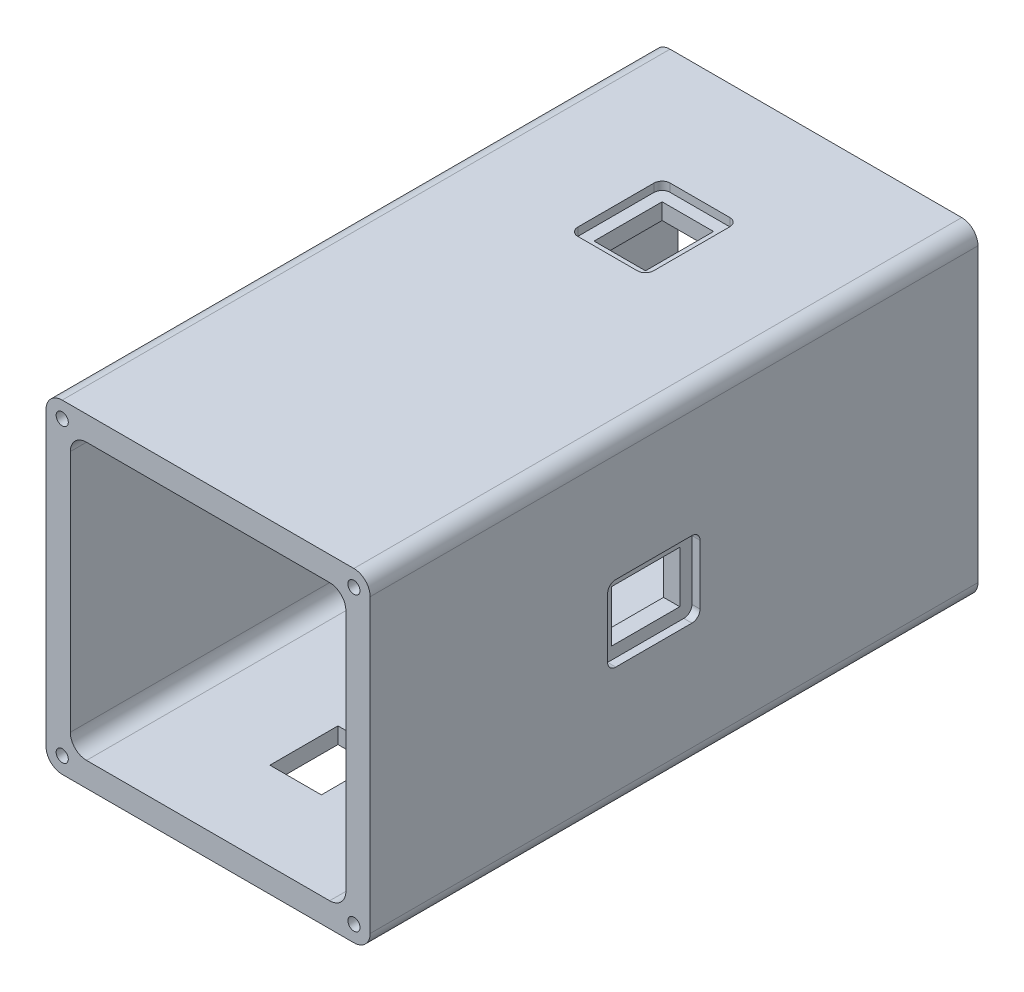
from build123d import *

# Parameters (mm, degrees)
BOSS_EXTRUDE1_DEPTH = 150
SKETCH2_R           = 1.500003704
SKETCH2_R_2         = 1.500002005
SKETCH2_R_3         = 1.500336032
SKETCH2_R_4         = 1.499979566
CUT_EXTRUDE1_DEPTH  = 5
SKETCH7_W           = 12.7
SKETCH7_H           = 16.8
CUT_EXTRUDE2_DEPTH  = 13
SKETCH8_W           = 16.8
SKETCH8_H           = 12.7
CUT_EXTRUDE3_DEPTH  = 13
SKETCH9_W           = 12.7
SKETCH9_H           = 16.8
CUT_EXTRUDE4_DEPTH  = 13
SKETCH10_W          = 18.7
SKETCH10_H          = 22.8
CUT_EXTRUDE5_DEPTH  = 2
FILLET1_R           = 2
SKETCH12_W          = 22.8
SKETCH12_H          = 18.7
CUT_EXTRUDE6_DEPTH  = 2
FILLET2_R           = 2
SKETCH13_W          = 18.7
SKETCH13_H          = 22.8
CUT_EXTRUDE7_DEPTH  = 2
FILLET3_R           = 2


with BuildPart() as part:
    # Sketch1 → Boss-Extrude1 (new body)
    with BuildSketch(Plane.XY):
        with BuildLine():
            Line((10.572650429, 43.57995567), (10.572650429, -28.420041122))
            ThreePointArc((10.572650429, -28.420041122), (11.744224426, -31.248470954), (14.572654257, -32.420044951))
            Line((14.572654257, -32.420044951), (86.572574673, -32.420044951))
            ThreePointArc((86.572574673, -32.420044951), (89.401092734, -31.248434409), (90.572703276, -28.419916348))
            Line((90.572703276, -28.419916348), (90.572703276, 43.558936727))
            ThreePointArc((90.572703276, 43.558936727), (89.3949748, 46.402224786), (86.551686742, 47.579953261))
            Line((86.551686742, 47.579953261), (14.57264802, 47.579953261))
            ThreePointArc((14.57264802, 47.579953261), (11.744222599, 46.408381091), (10.572650429, 43.57995567))
        make_face()
        with BuildLine():
            Line((16.572650429, 37.579953261), (16.572650429, -22.420044951))
            ThreePointArc((16.572650429, -22.420044951), (17.744223304, -25.248472075), (20.572650429, -26.420044951))
            Line((20.572650429, -26.420044951), (80.572648641, -26.420044951))
            ThreePointArc((80.572648641, -26.420044951), (83.401075766, -25.248472075), (84.572648641, -22.420044951))
            Line((84.572648641, -22.420044951), (84.572648641, 37.579953261))
            ThreePointArc((84.572648641, 37.579953261), (83.401075766, 40.408380386), (80.572648641, 41.579953261))
            Line((80.572648641, 41.579953261), (20.572650429, 41.579953261))
            ThreePointArc((20.572650429, 41.579953261), (17.744223304, 40.408380386), (16.572650429, 37.579953261))
        make_face(mode=Mode.SUBTRACT)
    extrude(amount=BOSS_EXTRUDE1_DEPTH)

    # Sketch2 → Cut-Extrude1 (cut)
    with BuildSketch(Plane.XY.offset(150)):
        with Locations((14.572654257, -28.420041122)):
            Circle(SKETCH2_R)
        with Locations((14.57264802, 43.57995567)):
            Circle(SKETCH2_R_2)
        with Locations((86.551686742, 43.558936727)):
            Circle(SKETCH2_R_3)
        with Locations((86.572574673, -28.419916348)):
            Circle(SKETCH2_R_4)
    cut_extrude1 = extrude(amount=-CUT_EXTRUDE1_DEPTH, mode=Mode.SUBTRACT)

    # Mirror1: Cut-Extrude1 across plane
    add(cut_extrude1.mirror(Plane(origin=(0, 0, 75), x_dir=(1, 0, 0), z_dir=(0, 0, -1))), mode=Mode.SUBTRACT)

    # Sketch7 → Cut-Extrude2 (cut)
    with BuildSketch(Plane(origin=(0, 47.579953261, 0), x_dir=(1, 0, 0), z_dir=(0, 1, 0))):
        with Locations((50.562167381, -40)):
            Rectangle(SKETCH7_W, SKETCH7_H)
    extrude(amount=-CUT_EXTRUDE2_DEPTH, mode=Mode.SUBTRACT)

    # Sketch8 → Cut-Extrude3 (cut)
    with BuildSketch(Plane(origin=(90.572703276, 0, 0), x_dir=(0, 0, -1), z_dir=(1, 0, 0))):
        with Locations((-80, 7.569510189)):
            Rectangle(SKETCH8_W, SKETCH8_H)
    extrude(amount=-CUT_EXTRUDE3_DEPTH, mode=Mode.SUBTRACT)

    # Sketch9 → Cut-Extrude4 (cut)
    with BuildSketch(Plane.XZ.offset(32.420044951)):
        with Locations((50.572614465, 120)):
            Rectangle(SKETCH9_W, SKETCH9_H)
    extrude(amount=-CUT_EXTRUDE4_DEPTH, mode=Mode.SUBTRACT)

    # Sketch10 → Cut-Extrude5 (cut)
    with BuildSketch(Plane(origin=(0, 47.579953261, 0), x_dir=(1, 0, 0), z_dir=(0, 1, 0))):
        with Locations((50.562167381, -40)):
            Rectangle(SKETCH10_W, SKETCH10_H)
    extrude(amount=-CUT_EXTRUDE5_DEPTH, mode=Mode.SUBTRACT)

    # Fillet1
    fillet1_edges = [part.edges().sort_by_distance(p)[0] for p in [
        (59.912167381, 46.579953261, 28.6),
        (59.912167381, 46.579953261, 51.4),
        (41.212167381, 46.579953261, 51.4),
        (41.212167381, 46.579953261, 28.6),
    ]]
    fillet(fillet1_edges, radius=FILLET1_R)

    # Sketch12 → Cut-Extrude6 (cut)
    with BuildSketch(Plane(origin=(90.572703276, 0, 0), x_dir=(0, 0, -1), z_dir=(1, 0, 0))):
        with Locations((-80, 7.569510189)):
            Rectangle(SKETCH12_W, SKETCH12_H)
    extrude(amount=-CUT_EXTRUDE6_DEPTH, mode=Mode.SUBTRACT)

    # Fillet2
    fillet2_edges = [part.edges().sort_by_distance(p)[0] for p in [
        (89.572703276, 16.919510189, 91.4),
        (89.572703276, 16.919510189, 68.6),
        (89.572703276, -1.780489811, 68.6),
        (89.572703276, -1.780489811, 91.4),
    ]]
    fillet(fillet2_edges, radius=FILLET2_R)

    # Sketch13 → Cut-Extrude7 (cut)
    with BuildSketch(Plane.XZ.offset(32.420044951)):
        with Locations((50.572614465, 120)):
            Rectangle(SKETCH13_W, SKETCH13_H)
    extrude(amount=-CUT_EXTRUDE7_DEPTH, mode=Mode.SUBTRACT)

    # Fillet3
    fillet3_edges = [part.edges().sort_by_distance(p)[0] for p in [
        (41.222614465, -31.420044951, 108.6),
        (41.222614465, -31.420044951, 131.4),
        (59.922614465, -31.420044951, 131.4),
        (59.922614465, -31.420044951, 108.6),
    ]]
    fillet(fillet3_edges, radius=FILLET3_R)


solid = part.part
